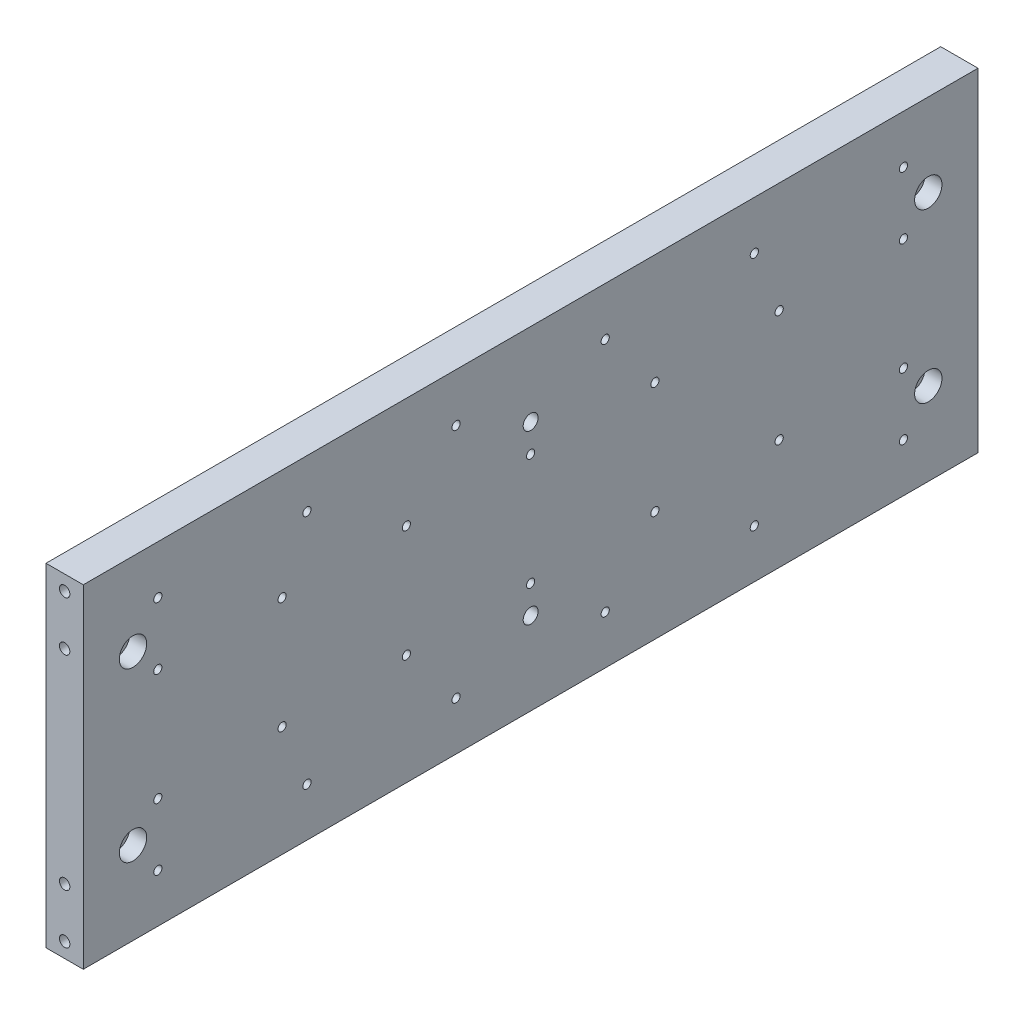
from build123d import *

# Parameters (mm, degrees)
SKETCH1_W                                            = 360
SKETCH1_H                                            = 134
BOSS_EXTRUDE1_DEPTH                                  = 15
M5_TAPPED_HOLE1_AT_2_COUNT                           = 2
M5_TAPPED_HOLE1_AT_2_PITCH                           = 122
M5_TAPPED_HOLE1_AT_3_COUNT                           = 2
M5_TAPPED_HOLE1_AT_3_PITCH                           = 102
M5_TAPPED_HOLE1_AT_4_COUNT                           = 2
M5_TAPPED_HOLE1_AT_4_PITCH                           = 20
M4_TAPPED_HOLE1_AT_2_COUNT                           = 2
M4_TAPPED_HOLE1_AT_2_PITCH                           = 45
LPATTERN1_COUNT                                      = 7
LPATTERN1_PITCH                                      = 50
M4_TAPPED_HOLE2_AT_2_COUNT                           = 2
M4_TAPPED_HOLE2_AT_2_PITCH                           = 95
LPATTERN2_COUNT                                      = 6
LPATTERN2_PITCH                                      = 60
M5_TAPPED_HOLE2_D                                    = 4.2
M5_TAPPED_HOLE2_DEPTH                                = 12.4
M5_TAPPED_HOLE2_TIP                                  = 1.2618073
M4_TAPPED_HOLE3_D                                    = 3.3
M4_TAPPED_HOLE3_DEPTH                                = 10.1
M4_TAPPED_HOLE3_TIP                                  = 0.991420021
CBORE_FOR_M6_HEXAGON_SOCKET_HEAD_CAP_SCR_D           = 6.6
CBORE_FOR_M6_HEXAGON_SOCKET_HEAD_CAP_SCR_CBORE_D     = 11
CBORE_FOR_M6_HEXAGON_SOCKET_HEAD_CAP_SCR_CBORE_DEPTH = 6.8
F_6_0MM_DOWEL_HOLE1_D                                = 6


with BuildPart() as part:
    # Sketch1 → Boss-Extrude1 (new body)
    with BuildSketch(Plane(origin=(0, 0, 0), x_dir=(0, 0, -1), z_dir=(1, 0, 0))):
        Rectangle(SKETCH1_W, SKETCH1_H)
    extrude(amount=BOSS_EXTRUDE1_DEPTH)

    # Sketch3 → M5 Tapped Hole1 (revolve, cut)
    with BuildSketch(Plane(origin=(7.5, -61, 180), x_dir=(0, -1, 0), z_dir=(1, 0, 0))):
        Polygon((0, 0), (0, 13.6618073), (2.1, 12.4), (2.1, 0), align=None)
    m5_tapped_hole1 = revolve(axis=Axis((7.5, -61, 186.35), (0, 0, -1)), mode=Mode.SUBTRACT)

    # M5 Tapped Hole1 at 2: M5 Tapped Hole1 ×2
    with Locations(*[(0, i * M5_TAPPED_HOLE1_AT_2_PITCH, 0) for i in range(1, M5_TAPPED_HOLE1_AT_2_COUNT)]):
        add(m5_tapped_hole1, mode=Mode.SUBTRACT)

    # M5 Tapped Hole1 at 3: M5 Tapped Hole1 ×2
    with Locations(*[(0, i * M5_TAPPED_HOLE1_AT_3_PITCH, 0) for i in range(1, M5_TAPPED_HOLE1_AT_3_COUNT)]):
        add(m5_tapped_hole1, mode=Mode.SUBTRACT)

    # M5 Tapped Hole1 at 4: M5 Tapped Hole1 ×2
    with Locations(*[(0, i * M5_TAPPED_HOLE1_AT_4_PITCH, 0) for i in range(1, M5_TAPPED_HOLE1_AT_4_COUNT)]):
        add(m5_tapped_hole1, mode=Mode.SUBTRACT)

    # Mirror1: M5 Tapped Hole1 across plane
    add(m5_tapped_hole1.mirror(Plane.XY), mode=Mode.SUBTRACT)

    # Mirror1 copy 1 sketch → Mirror1 copy 1 (revolve, cut)
    with BuildSketch(Plane(origin=(7.5, 61, -180), x_dir=(0, -1, 0), z_dir=(1, 0, 0))):
        Polygon((0, 0), (0, -13.6618073), (2.1, -12.4), (2.1, 0), align=None)
    revolve(axis=Axis((7.5, 61, -186.35), (0, 0, -1)), mode=Mode.SUBTRACT)

    # Mirror1 copy 2 sketch → Mirror1 copy 2 (revolve, cut)
    with BuildSketch(Plane(origin=(7.5, 41, -180), x_dir=(0, -1, 0), z_dir=(1, 0, 0))):
        Polygon((0, 0), (0, -13.6618073), (2.1, -12.4), (2.1, 0), align=None)
    revolve(axis=Axis((7.5, 41, -186.35), (0, 0, -1)), mode=Mode.SUBTRACT)

    # Mirror1 copy 3 sketch → Mirror1 copy 3 (revolve, cut)
    with BuildSketch(Plane(origin=(7.5, -41, -180), x_dir=(0, -1, 0), z_dir=(1, 0, 0))):
        Polygon((0, 0), (0, -13.6618073), (2.1, -12.4), (2.1, 0), align=None)
    revolve(axis=Axis((7.5, -41, -186.35), (0, 0, -1)), mode=Mode.SUBTRACT)

    # Sketch5 → M4 Tapped Hole1 (revolve, cut)
    with BuildSketch(Plane(origin=(15, 22.5, -150), x_dir=(0, 0, -1), z_dir=(0, 1, 0))):
        Polygon((0, 0), (0, 11.091420021), (1.65, 10.1), (1.65, 0), align=None)
    m4_tapped_hole1 = revolve(axis=Axis((21.35, 22.5, -150), (-1, 0, 0)), mode=Mode.SUBTRACT)

    # M4 Tapped Hole1 at 2: M4 Tapped Hole1 ×2
    with Locations(*[(0, -i * M4_TAPPED_HOLE1_AT_2_PITCH, 0) for i in range(1, M4_TAPPED_HOLE1_AT_2_COUNT)]):
        add(m4_tapped_hole1, mode=Mode.SUBTRACT)

    # LPattern1: M4 Tapped Hole1 ×7
    with Locations(*[(0, 0, i * LPATTERN1_PITCH) for i in range(1, LPATTERN1_COUNT)]):
        add(m4_tapped_hole1, mode=Mode.SUBTRACT)

    # LPattern1 copy 1 sketch → LPattern1 copy 1 (revolve, cut)
    with BuildSketch(Plane(origin=(15, -22.5, -100), x_dir=(0, 0, -1), z_dir=(0, 1, 0))):
        Polygon((0, 0), (0, 11.091420021), (1.65, 10.1), (1.65, 0), align=None)
    revolve(axis=Axis((21.35, -22.5, -100), (-1, 0, 0)), mode=Mode.SUBTRACT)

    # LPattern1 copy 2 sketch → LPattern1 copy 2 (revolve, cut)
    with BuildSketch(Plane(origin=(15, -22.5, -50), x_dir=(0, 0, -1), z_dir=(0, 1, 0))):
        Polygon((0, 0), (0, 11.091420021), (1.65, 10.1), (1.65, 0), align=None)
    revolve(axis=Axis((21.35, -22.5, -50), (-1, 0, 0)), mode=Mode.SUBTRACT)

    # LPattern1 copy 3 sketch → LPattern1 copy 3 (revolve, cut)
    with BuildSketch(Plane(origin=(15, -22.5, 0), x_dir=(0, 0, -1), z_dir=(0, 1, 0))):
        Polygon((0, 0), (0, 11.091420021), (1.65, 10.1), (1.65, 0), align=None)
    revolve(axis=Axis((21.35, -22.5, 0), (-1, 0, 0)), mode=Mode.SUBTRACT)

    # LPattern1 copy 4 sketch → LPattern1 copy 4 (revolve, cut)
    with BuildSketch(Plane(origin=(15, -22.5, 50), x_dir=(0, 0, -1), z_dir=(0, 1, 0))):
        Polygon((0, 0), (0, 11.091420021), (1.65, 10.1), (1.65, 0), align=None)
    revolve(axis=Axis((21.35, -22.5, 50), (-1, 0, 0)), mode=Mode.SUBTRACT)

    # LPattern1 copy 5 sketch → LPattern1 copy 5 (revolve, cut)
    with BuildSketch(Plane(origin=(15, -22.5, 100), x_dir=(0, 0, -1), z_dir=(0, 1, 0))):
        Polygon((0, 0), (0, 11.091420021), (1.65, 10.1), (1.65, 0), align=None)
    revolve(axis=Axis((21.35, -22.5, 100), (-1, 0, 0)), mode=Mode.SUBTRACT)

    # LPattern1 copy 6 sketch → LPattern1 copy 6 (revolve, cut)
    with BuildSketch(Plane(origin=(15, -22.5, 150), x_dir=(0, 0, -1), z_dir=(0, 1, 0))):
        Polygon((0, 0), (0, 11.091420021), (1.65, 10.1), (1.65, 0), align=None)
    revolve(axis=Axis((21.35, -22.5, 150), (-1, 0, 0)), mode=Mode.SUBTRACT)

    # Sketch7 → M4 Tapped Hole2 (revolve, cut)
    with BuildSketch(Plane(origin=(15, 47.5, -150), x_dir=(0, 0, -1), z_dir=(0, 1, 0))):
        Polygon((0, 0), (0, 11.091420021), (1.65, 10.1), (1.65, 0), align=None)
    m4_tapped_hole2 = revolve(axis=Axis((21.35, 47.5, -150), (-1, 0, 0)), mode=Mode.SUBTRACT)

    # M4 Tapped Hole2 at 2: M4 Tapped Hole2 ×2
    with Locations(*[(0, -i * M4_TAPPED_HOLE2_AT_2_PITCH, 0) for i in range(1, M4_TAPPED_HOLE2_AT_2_COUNT)]):
        add(m4_tapped_hole2, mode=Mode.SUBTRACT)

    # LPattern2: M4 Tapped Hole2 ×6
    with Locations(*[(0, 0, i * LPATTERN2_PITCH) for i in range(1, LPATTERN2_COUNT)]):
        add(m4_tapped_hole2, mode=Mode.SUBTRACT)

    # LPattern2 copy 1 sketch → LPattern2 copy 1 (revolve, cut)
    with BuildSketch(Plane(origin=(15, -47.5, -90), x_dir=(0, 0, -1), z_dir=(0, 1, 0))):
        Polygon((0, 0), (0, 11.091420021), (1.65, 10.1), (1.65, 0), align=None)
    revolve(axis=Axis((21.35, -47.5, -90), (-1, 0, 0)), mode=Mode.SUBTRACT)

    # LPattern2 copy 2 sketch → LPattern2 copy 2 (revolve, cut)
    with BuildSketch(Plane(origin=(15, -47.5, -30), x_dir=(0, 0, -1), z_dir=(0, 1, 0))):
        Polygon((0, 0), (0, 11.091420021), (1.65, 10.1), (1.65, 0), align=None)
    revolve(axis=Axis((21.35, -47.5, -30), (-1, 0, 0)), mode=Mode.SUBTRACT)

    # LPattern2 copy 3 sketch → LPattern2 copy 3 (revolve, cut)
    with BuildSketch(Plane(origin=(15, -47.5, 30), x_dir=(0, 0, -1), z_dir=(0, 1, 0))):
        Polygon((0, 0), (0, 11.091420021), (1.65, 10.1), (1.65, 0), align=None)
    revolve(axis=Axis((21.35, -47.5, 30), (-1, 0, 0)), mode=Mode.SUBTRACT)

    # LPattern2 copy 4 sketch → LPattern2 copy 4 (revolve, cut)
    with BuildSketch(Plane(origin=(15, -47.5, 90), x_dir=(0, 0, -1), z_dir=(0, 1, 0))):
        Polygon((0, 0), (0, 11.091420021), (1.65, 10.1), (1.65, 0), align=None)
    revolve(axis=Axis((21.35, -47.5, 90), (-1, 0, 0)), mode=Mode.SUBTRACT)

    # LPattern2 copy 5 sketch → LPattern2 copy 5 (revolve, cut)
    with BuildSketch(Plane(origin=(15, -47.5, 150), x_dir=(0, 0, -1), z_dir=(0, 1, 0))):
        Polygon((0, 0), (0, 11.091420021), (1.65, 10.1), (1.65, 0), align=None)
    revolve(axis=Axis((21.35, -47.5, 150), (-1, 0, 0)), mode=Mode.SUBTRACT)

    # M5 Tapped Hole2
    with Locations(Plane.ZY):
        with Locations((-142.5, 58), (-117.5, 58), (32.5, 58), (57.5, 58)):
            Hole(M5_TAPPED_HOLE2_D / 2, depth=M5_TAPPED_HOLE2_DEPTH)
            with Locations((0, 0, -(M5_TAPPED_HOLE2_DEPTH + M5_TAPPED_HOLE2_TIP / 2))):  # 118° drill point
                Cone(0, M5_TAPPED_HOLE2_D / 2, M5_TAPPED_HOLE2_TIP, mode=Mode.SUBTRACT)

    # M4 Tapped Hole3
    with Locations(Plane.ZY):
        with Locations((-172.5, 59.6), (87.5, 59.6), (2.5, 59.6), (-87.5, 59.6)):
            Hole(M4_TAPPED_HOLE3_D / 2, depth=M4_TAPPED_HOLE3_DEPTH)
            with Locations((0, 0, -(M4_TAPPED_HOLE3_DEPTH + M4_TAPPED_HOLE3_TIP / 2))):  # 118° drill point
                Cone(0, M4_TAPPED_HOLE3_D / 2, M4_TAPPED_HOLE3_TIP, mode=Mode.SUBTRACT)

    # CBORE for M6 Hexagon socket head cap screws1 (through all)
    with Locations(Plane(origin=(15, 0, 0), x_dir=(0, 0, -1), z_dir=(1, 0, 0))):
        with Locations((-160, 33.75), (-160, -33.75), (160, -33.75), (160, 33.75)):
            CounterBoreHole(CBORE_FOR_M6_HEXAGON_SOCKET_HEAD_CAP_SCR_D / 2, CBORE_FOR_M6_HEXAGON_SOCKET_HEAD_CAP_SCR_CBORE_D / 2, CBORE_FOR_M6_HEXAGON_SOCKET_HEAD_CAP_SCR_CBORE_DEPTH)

    # Ø6.0mm dowel hole1 (through all)
    with Locations(Plane(origin=(15, 0, 0), x_dir=(0, 0, -1), z_dir=(1, 0, 0))):
        with Locations((0, -33.75), (0, 33.75)):
            Hole(F_6_0MM_DOWEL_HOLE1_D / 2)


solid = part.part
